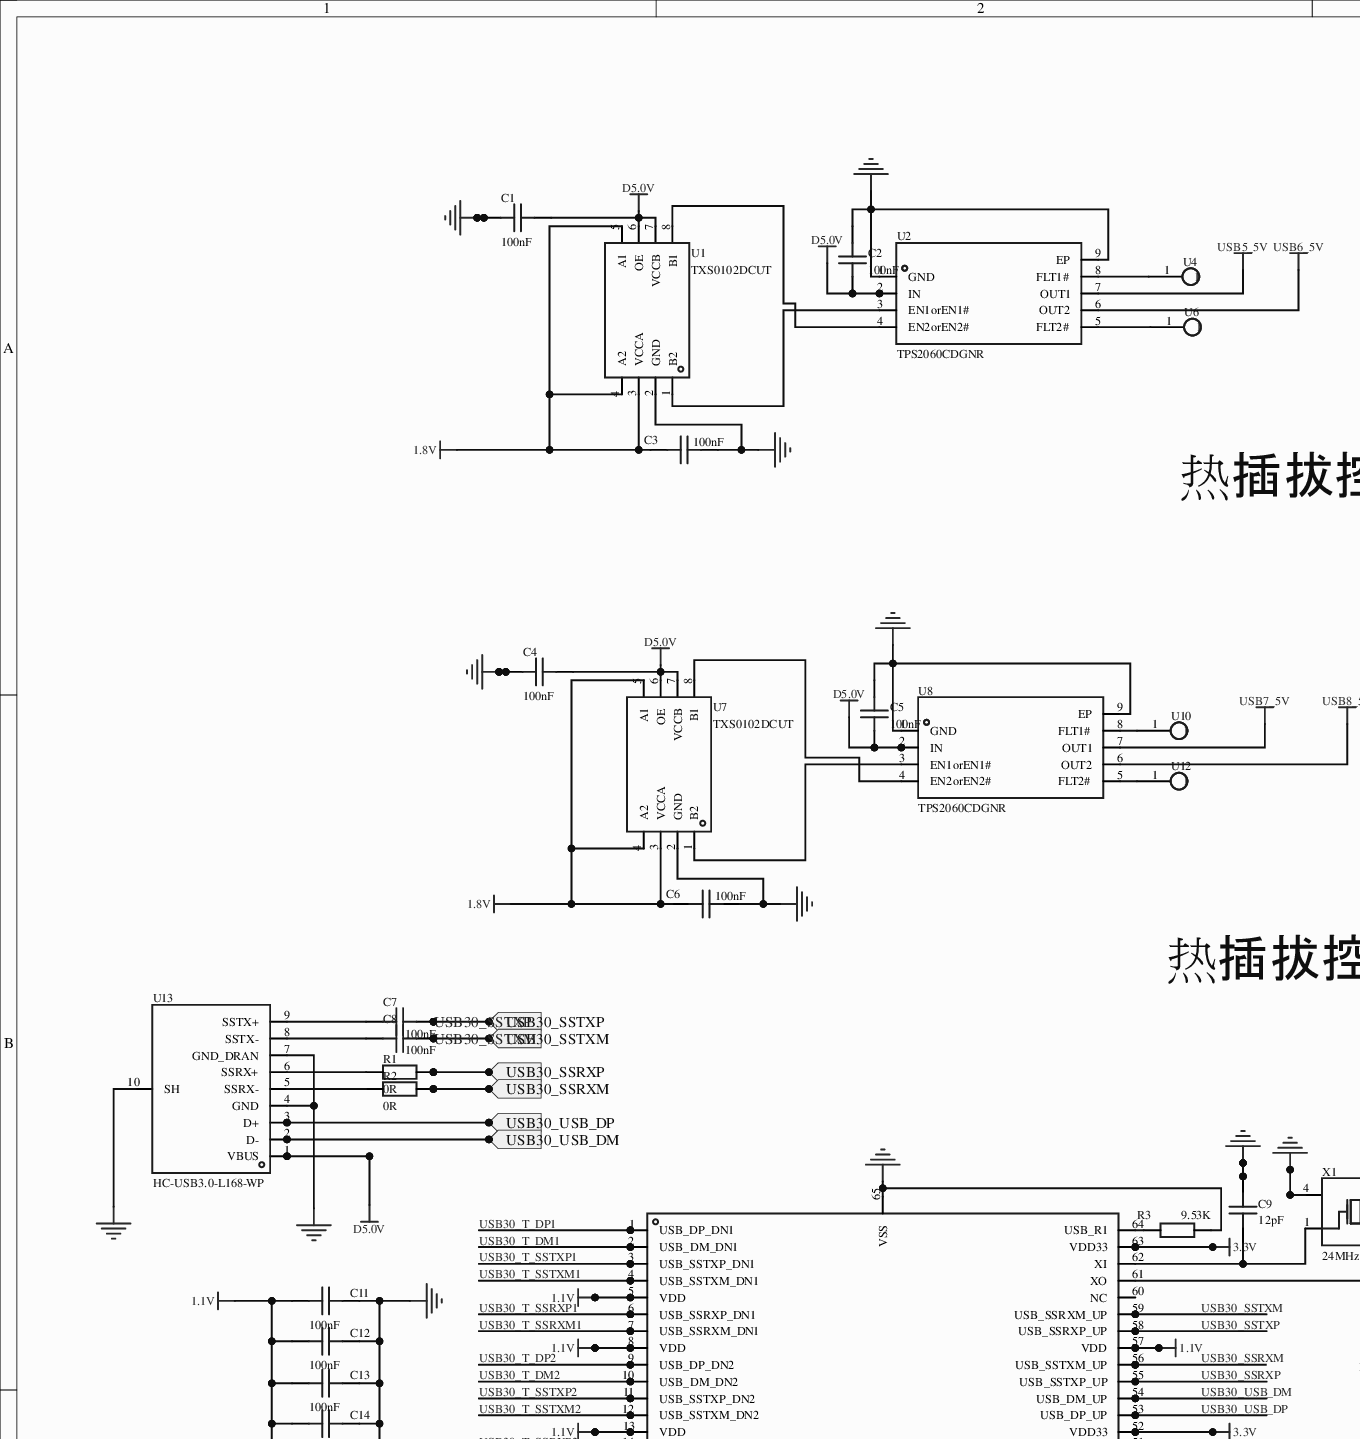
[diagram p0: MISC51972-3.schdoc, top left]
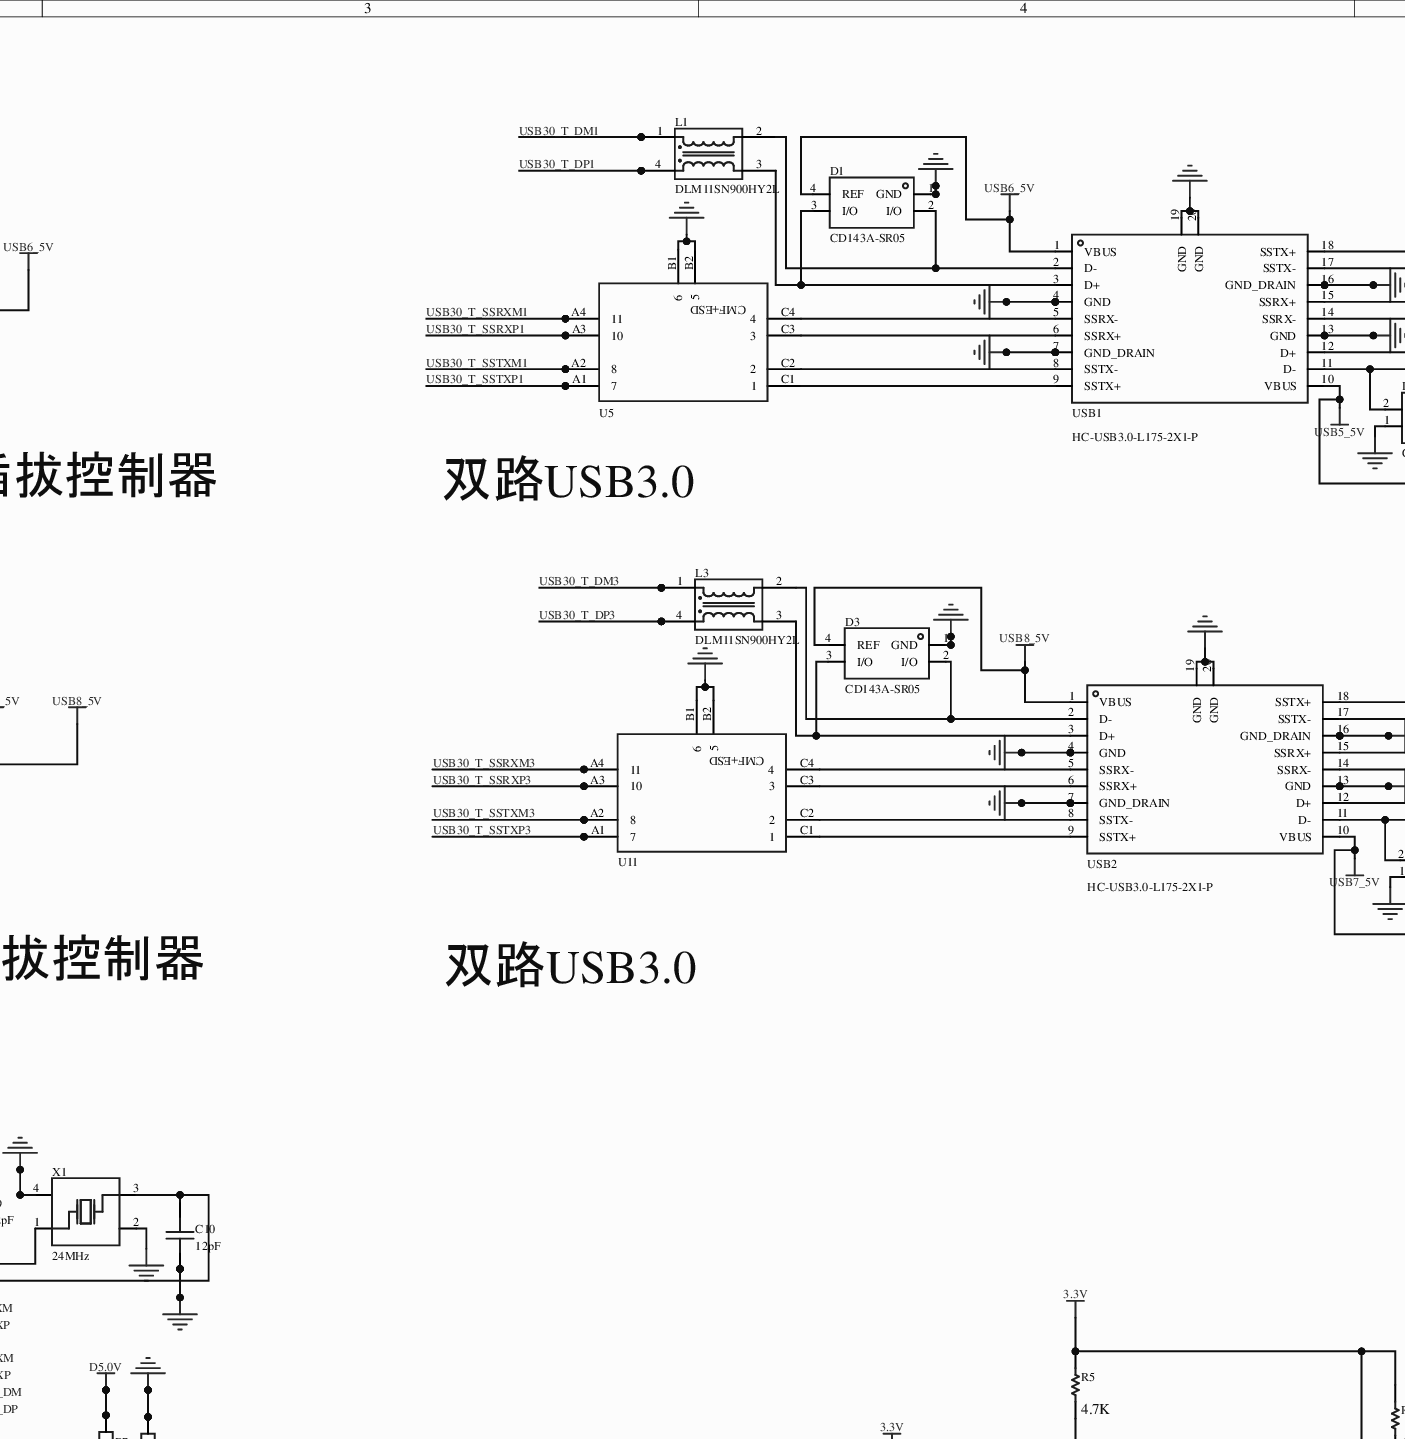
[diagram p1: MISC51972-3.schdoc, top middle]
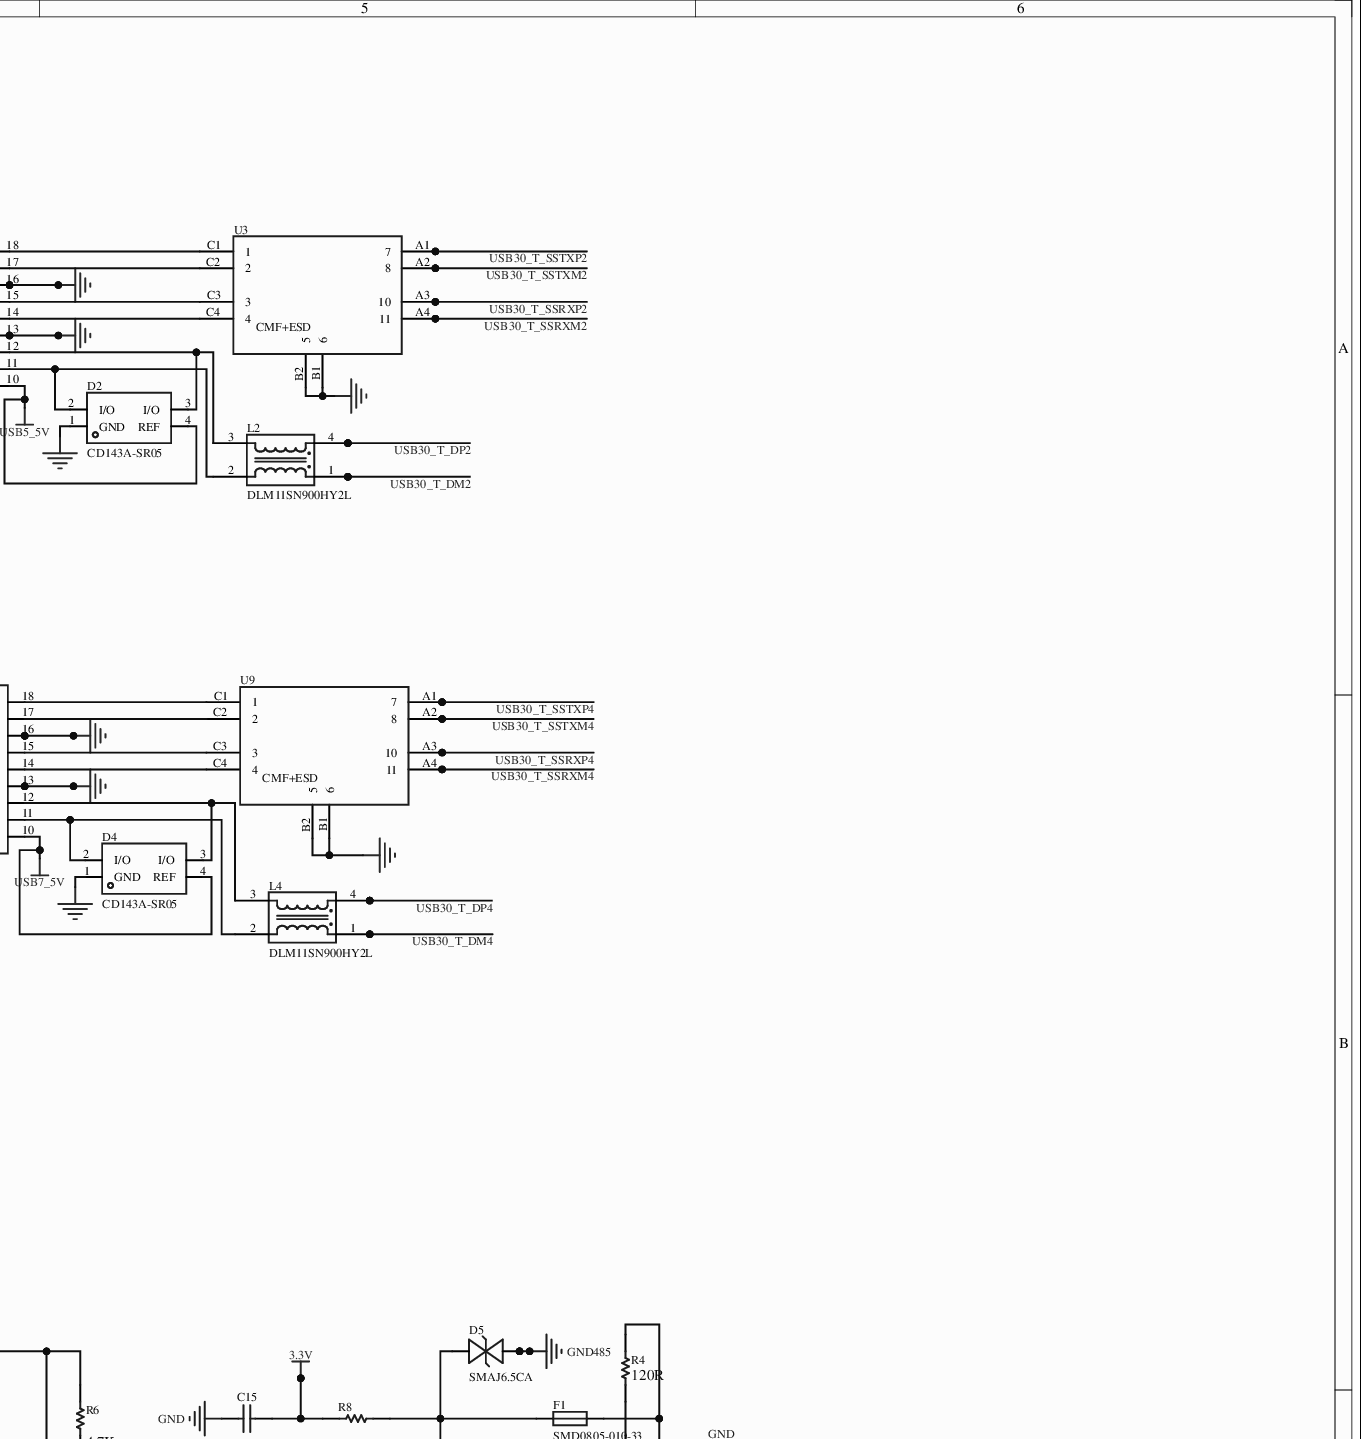
[diagram p2: MISC51972-3.schdoc, top right]
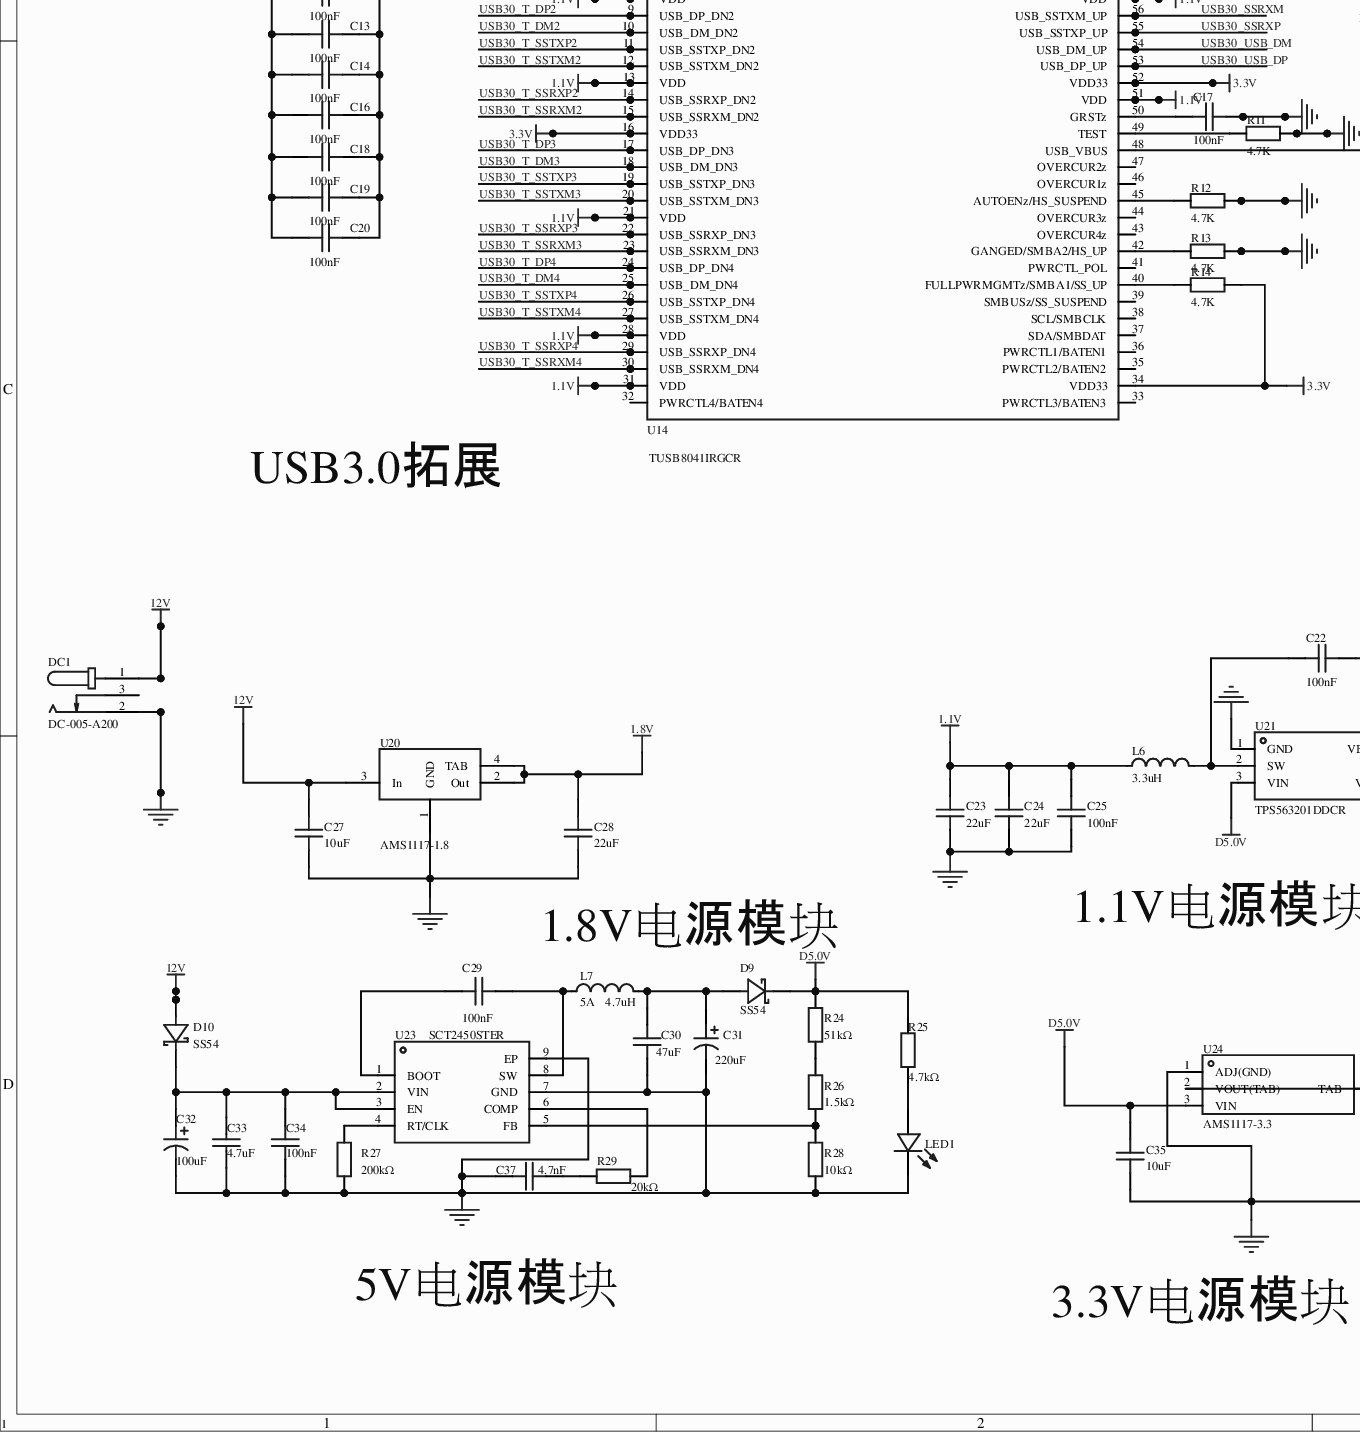
[diagram p3: MISC51972-3.schdoc, bottom left]
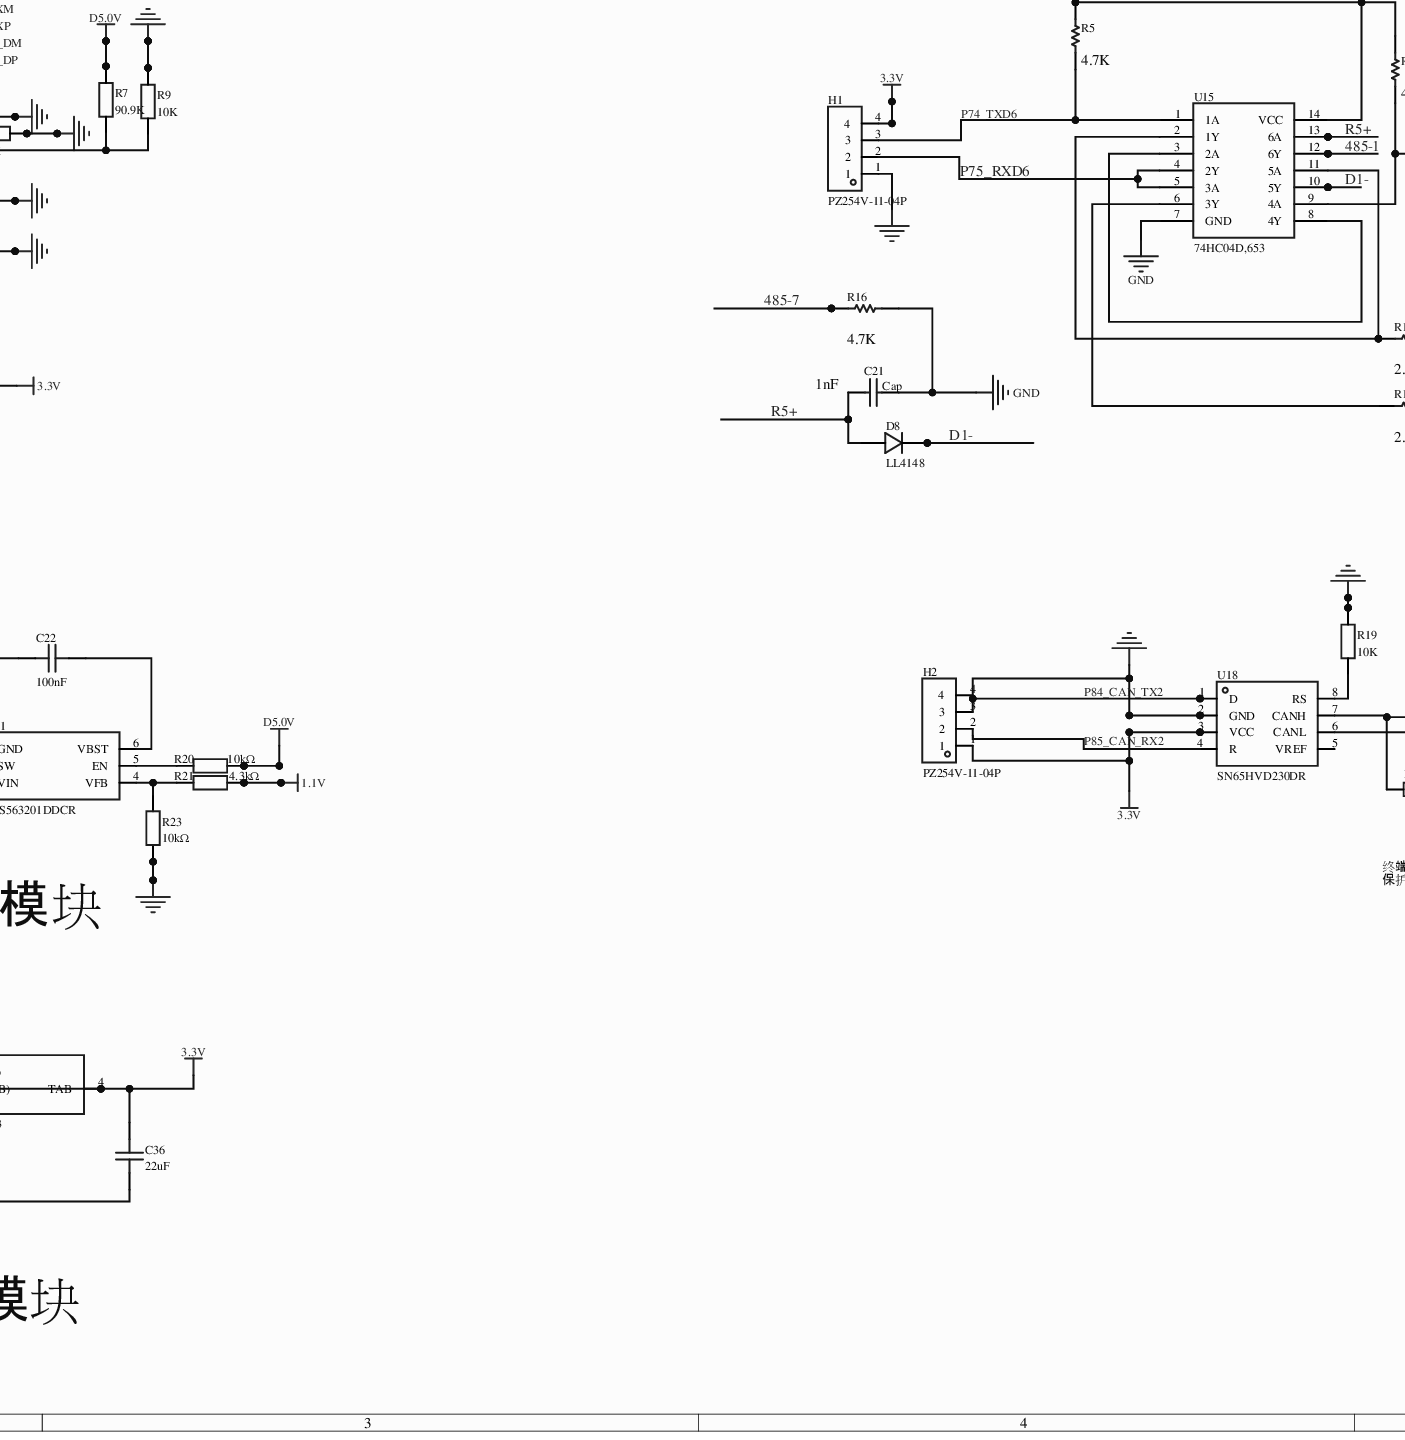
[diagram p4: MISC51972-3.schdoc, bottom middle]
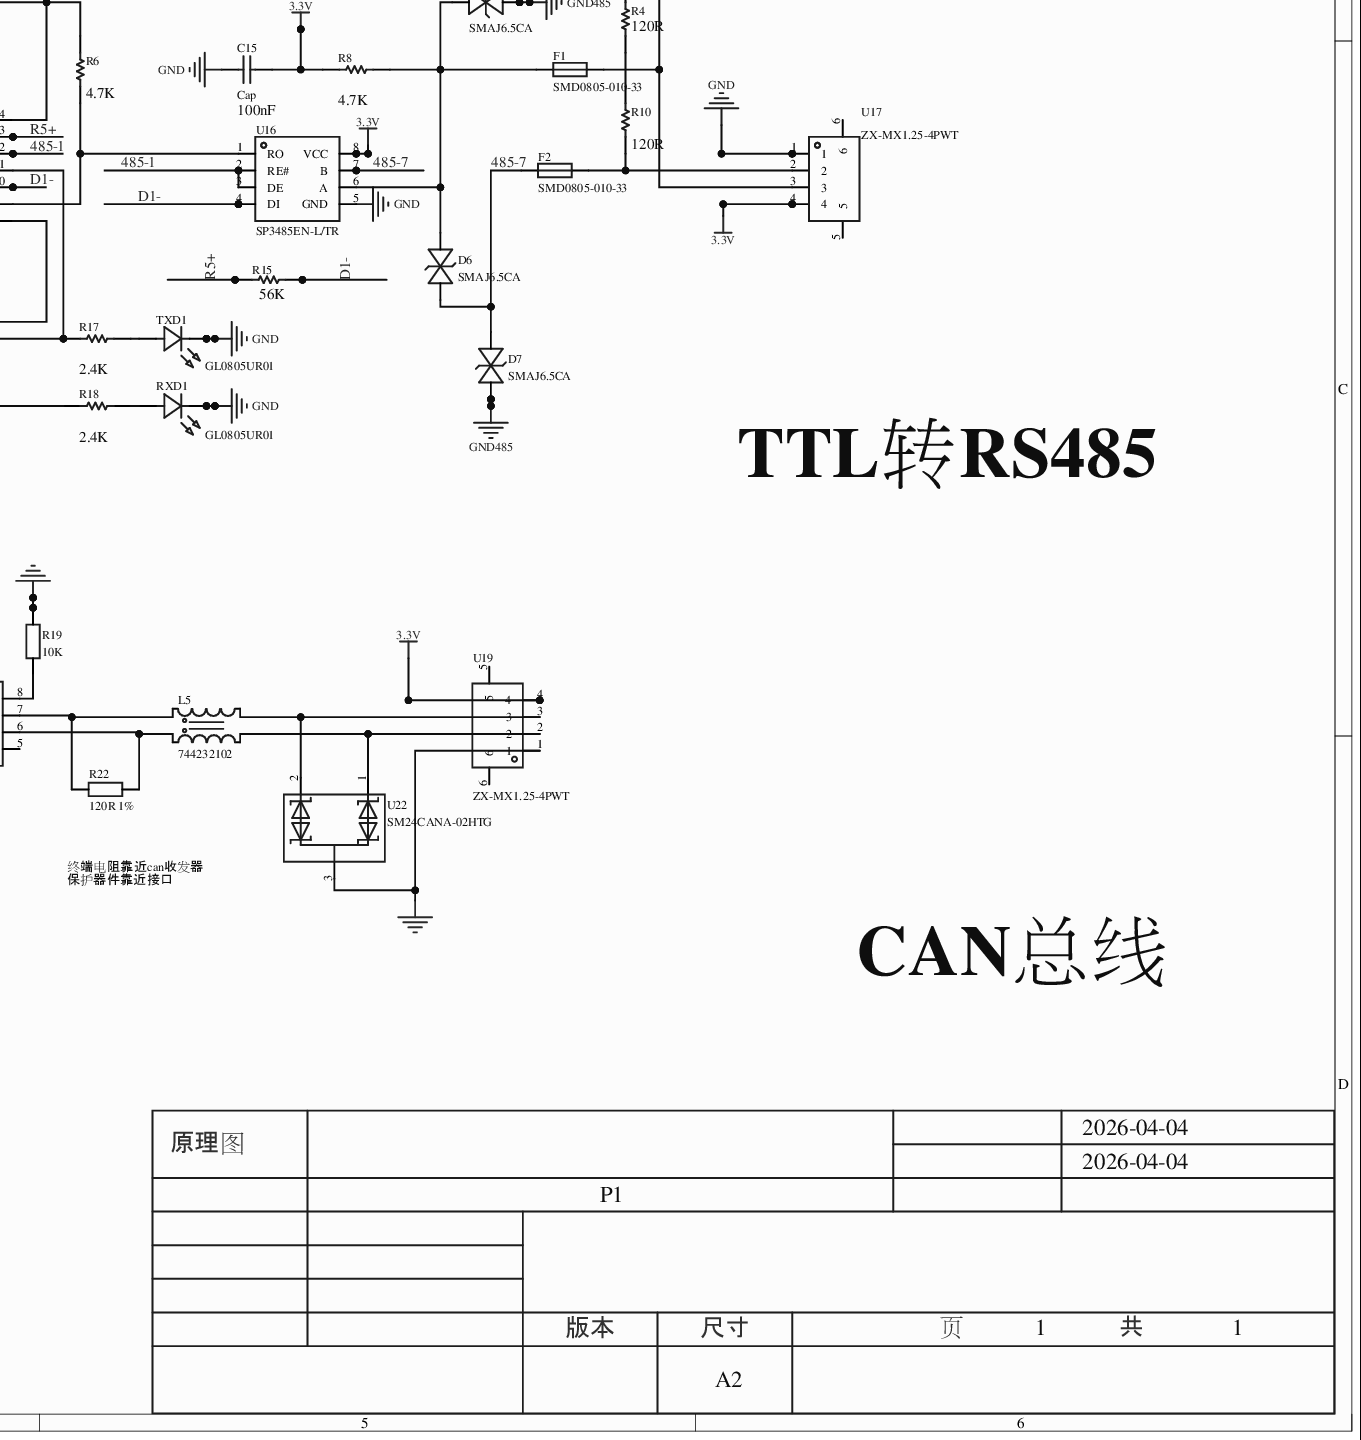
[diagram p5: MISC51972-3.schdoc, bottom right]
# Altium project MISC51972-2.PrjPcb (part 1 of 3)
1 sheet, 117 parts. Net scope: flat (ports and power ports of the same name join across sheets).
Board file: MISC51972.pcbdoc